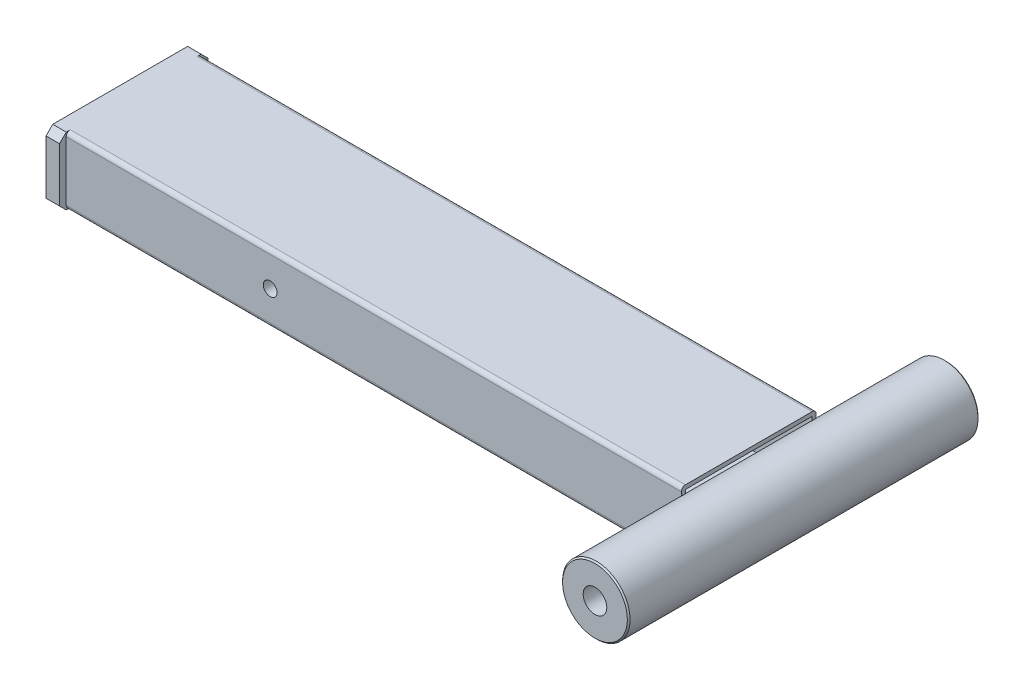
SolidWorks part; units mm, degrees
material "1023 碳钢板 (SS)"
ref_plane "前视基准面" through (0, 0, 0) normal (0, 0, 1) x (1, 0, 0)
ref_plane "上视基准面" through (0, 0, 0) normal (0, 1, 0) x (1, 0, 0)
ref_plane "右视基准面" through (0, 0, 0) normal (1, 0, 0) x (0, 0, -1)
ref_plane "基准面4" through (0, 25, 0) normal (0, 1, 0) x (1, 0, 0)
sketch "草图1" plane through (0, 25, 0) normal (0, 1, 0) x (1, 0, 0)
  line L0 (228, -55) -> (228, 55)
  line L1 (228, 55) -> (-238, 55)
  line L2 (-238, 55) -> (-238, -55)
  line L3 (-238, -55) -> (228, -55)
extrude "凸台-拉伸1" add sketch "草图1" against normal blind 50
sketch "草图2" plane through (0, -25, 0) normal (0, -1, 0) x (1, 0, 0)
  line L0 (228, -55) -> (228, -50)
  line L1 (228, -50) -> (-228, -50)
  line L2 (-228, -50) -> (-228, -55)
  line L3 (-228, -55) -> (228, -55)
extrude "切除-拉伸1" cut sketch "草图2" against normal through all
sketch "草图3" plane through (0, -25, 0) normal (0, -1, 0) x (1, 0, 0)
  line L0 (-228, 50) -> (228, 50)
  line L1 (228, 50) -> (228, 55)
  line L2 (228, 55) -> (-228, 55)
  line L3 (-228, 55) -> (-228, 50)
extrude "切除-拉伸2" cut sketch "草图3" against normal through all
sketch "草图4" plane through (228, 0, 0) normal (1, 0, 0) x (0, 0, -1)
  line L0 (-47, -22) -> (47, -22)
  line L1 (47, -22) -> (47, 22)
  line L2 (47, 22) -> (-47, 22)
  line L3 (-47, 22) -> (-47, -22)
  line L4 (-50, 25) -> (50, 25) construction
extrude "切除-拉伸3" cut sketch "草图4" against normal blind 456
ref_plane "基准面5" through (0, 0, 0) normal (0, -1, 0) x (1, 0, 0)
sketch "草图5" plane through (0, 0, 0) normal (0, -1, 0) x (1, 0, 0)
  line L0 (-66.8, 47) -> (-76.8, 47)
  line L1 (-76.8, 47) -> (-76.8, -47)
  line L2 (-76.8, -47) -> (-66.8, -47)
  line L3 (-66.8, -47) -> (-66.8, 47)
  line L4 (-76.8, 47) -> (-76.8, -47) construction
  line L5 (228, 50) -> (228, -50) construction
revolve "旋转1" add sketch "草图5" angle 360 about L4
sketch "草图6" plane through (0, 0, 0) normal (0, 1, 0) x (1, 0, 0)
  line L0 (244, 130) -> (219, 130)
  line L1 (219, 130) -> (219, -130)
  line L2 (219, -130) -> (244, -130)
  line L3 (244, -130) -> (244, 130)
  line L4 (244, -130) -> (244, 130) construction
revolve "旋转2" add sketch "草图6" angle 360 about L4
hole_wizard "Ø8.5 (8.5) 直径孔1" positions "草图8" profile "草图7" hole size "Ø8.5" standard "ANSI Metric"
sketch "草图8" plane through (-228, 0, 0) normal (1, 0, 0) x (0, 0, -1)
  point P0 (40, 10)
  point P1 (-40, 10)
sketch "草图7" plane through (-228, 10, -40) normal (0, 1, 0) x (0, 0, -1)
  line L0 (0, 0) -> (0, 10)
  line L1 (0, 10) -> (4.25, 10)
  line L2 (4.25, 10) -> (4.25, 0)
  line L5 (4.25, 0) -> (0, 0)
  line L11 (0, -6.35) -> (0, 107.95) construction
  dimension "通孔孔直径" = 8.5
  dimension "通孔孔深度" = 10
sketch "草图24" plane through (0, 0, 50) normal (0, 0, 1) x (1, 0, 0)
  circle A0 centre (-76.8, 0) radius 18.4105
  circle A1 centre (244, 0) radius 25 construction
  dimension "D1" = 320.8
hole_wizard "M12 螺纹孔3" positions "草图27" profile "草图28" tap size "M12" standard "GB"
sketch "草图27" plane through (0, 0, 50) normal (0, 0, 1) x (1, 0, 0)
  point P0 (-76.8, 0)
sketch "草图28" plane through (-76.8, 0, 50) normal (1, 0, 0) x (0, -1, 0)
  line L0 (0, 0) -> (0, 32.3144)
  line L1 (0, 32.3144) -> (5.1, 29.25)
  line L2 (5.1, 29.25) -> (5.1, 0)
  line L5 (5.1, 0) -> (0, 0)
  line L10 (0, 32.3144) -> (-5.1, 29.25) construction
  line L11 (0, -6.35) -> (0, 107.95) construction
  dimension "螺纹孔钻头直径" = 10.2
  dimension "螺纹孔钻头深度" = 29.25
  dimension "导头角度" = 118
cosmetic thread "孔螺蚊线3" parameters "D1"=24, "D2"=12
sketch "草图29" plane through (0, 0, -50) normal (0, 0, -1) x (-1, 0, 0)
  circle A0 centre (76.8, 0) radius 12.1759
  circle A1 centre (-244, 0) radius 25 construction
  dimension "D1" = 320.8
hole_wizard "M12 螺纹孔4" positions "草图30" profile "草图31" tap size "M12" standard "GB"
sketch "草图30" plane through (0, 0, -50) normal (0, 0, -1) x (-1, 0, 0)
  point P0 (76.8, 0)
sketch "草图31" plane through (-76.8, 0, -50) normal (1, 0, 0) x (0, 1, 0)
  line L0 (0, 0) -> (0, 32.3144)
  line L1 (0, 32.3144) -> (5.1, 29.25)
  line L2 (5.1, 29.25) -> (5.1, 0)
  line L5 (5.1, 0) -> (0, 0)
  line L10 (0, 32.3144) -> (-5.1, 29.25) construction
  line L11 (0, -6.35) -> (0, 107.95) construction
  dimension "螺纹孔钻头直径" = 10.2
  dimension "螺纹孔钻头深度" = 29.25
  dimension "导头角度" = 118
cosmetic thread "孔螺蚊线4" parameters "D1"=24, "D2"=12
hole_wizard "Ø10.2 (10.2) 直径孔2" positions "草图12" profile "草图11" hole size "Ø10.2" standard "ANSI Metric"
sketch "草图12" plane through (0, 0, -50) normal (0, 0, -1) x (-1, 0, 0)
  point P0 (76.8, 0)
sketch "草图11" plane through (-76.8, 0, -50) normal (1, 0, 0) x (0, 1, 0)
  line L0 (0, 0) -> (0, 32.3144)
  line L1 (0, 32.3144) -> (5.1, 29.25)
  line L2 (5.1, 29.25) -> (5.1, 0)
  line L5 (5.1, 0) -> (0, 0)
  line L10 (0, 32.3144) -> (-5.1, 29.25) construction
  line L11 (0, -6.35) -> (0, 107.95) construction
  dimension "孔直径" = 10.2
  dimension "孔深度" = 29.25
  dimension "导头角度" = 118
chamfer "倒角1" distance 1 angle 45 2 edges at (219, 0, -130) (219, 0, 130)
fillet "圆角1" radius 3 4 edges at (0, -25, -50) (0, -25, 50) (0, 25, -50) (0, 25, 50)
chamfer "倒角2" distance 5 angle 45 4 edges at (-233, -25, -55) (-233, -25, 55) (-233, 25, 55) (-233, 25, -55)
sketch "草图34" plane through (0, 0, 130) normal (0, 0, 1) x (1, 0, 0)
  circle A0 centre (244, 0) radius 10.3312
hole_wizard "M20 螺纹孔1" positions "草图35" profile "草图36" tap size "M20" standard "GB"
sketch "草图35" plane through (0, 0, 130) normal (0, 0, 1) x (1, 0, 0)
  point P0 (244, 0)
sketch "草图36" plane through (244, 0, 130) normal (1, 0, 0) x (0, -1, 0)
  line L0 (0, 0) -> (0, 52.7575)
  line L1 (0, 52.7575) -> (8.75, 47.5)
  line L2 (8.75, 47.5) -> (8.75, 0)
  line L5 (8.75, 0) -> (0, 0)
  line L10 (0, 52.7575) -> (-8.75, 47.5) construction
  line L11 (0, -6.35) -> (0, 107.95) construction
  dimension "螺纹孔钻头直径" = 17.5
  dimension "螺纹孔钻头深度" = 47.5
  dimension "导头角度" = 118
cosmetic thread "孔螺蚊线5" parameters "D1"=40, "D2"=20
sketch "草图37" plane through (0, 0, -130) normal (0, 0, -1) x (-1, 0, 0)
  circle A0 centre (-244, 0) radius 9.4117
hole_wizard "M20 螺纹孔2" positions "草图38" profile "草图39" tap size "M20" standard "GB"
sketch "草图38" plane through (0, 0, -130) normal (0, 0, -1) x (-1, 0, 0)
  point P0 (-244, 0)
sketch "草图39" plane through (244, 0, -130) normal (1, 0, 0) x (0, 1, 0)
  line L0 (0, 0) -> (0, 52.7575)
  line L1 (0, 52.7575) -> (8.75, 47.5)
  line L2 (8.75, 47.5) -> (8.75, 0)
  line L5 (8.75, 0) -> (0, 0)
  line L10 (0, 52.7575) -> (-8.75, 47.5) construction
  line L11 (0, -6.35) -> (0, 107.95) construction
  dimension "螺纹孔钻头直径" = 17.5
  dimension "螺纹孔钻头深度" = 47.5
  dimension "导头角度" = 118
cosmetic thread "孔螺蚊线6" parameters "D1"=40, "D2"=20
